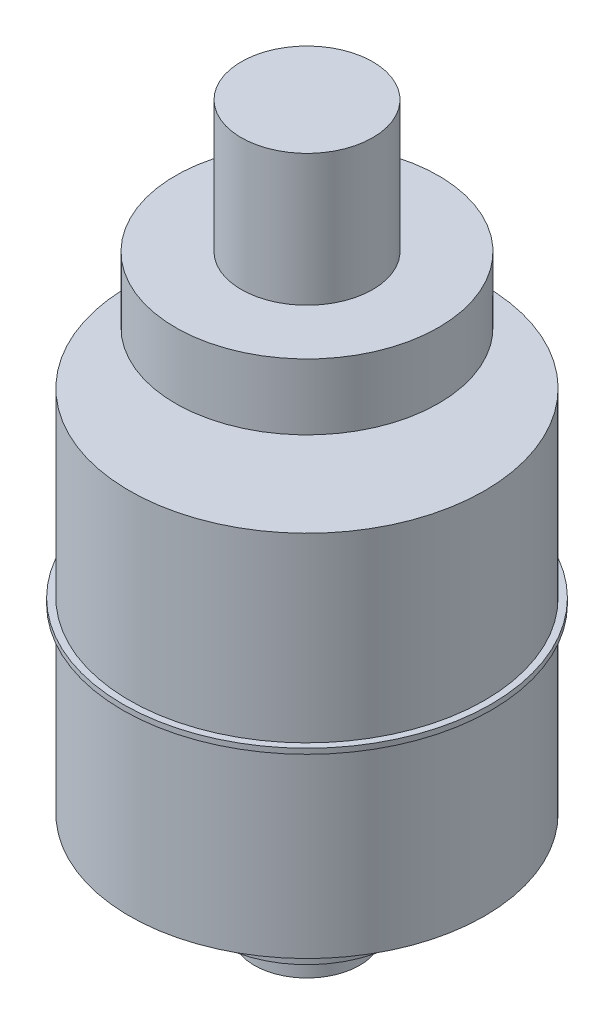
SolidWorks part; units mm, degrees
material "LY12#"
ref_plane "Front Plane" through (0, 0, 0) normal (0, 0, 1) x (1, 0, 0)
ref_plane "Top Plane" through (0, 0, 0) normal (0, 1, 0) x (1, 0, 0)
ref_plane "Right Plane" through (0, 0, 0) normal (1, 0, 0) x (0, 0, -1)
sketch "Sketch1" plane through (0, 0, 0) normal (0, 0, 1) x (1, 0, 0)
  line L0 (0, 0) -> (0, 55) construction
  line L1 (0, 55) -> (-5, 55)
  line L2 (-5, 55) -> (-5, 45)
  line L3 (-5, 45) -> (-10, 45)
  line L4 (-10, 45) -> (-10, 40)
  line L5 (-10, 40) -> (-4, 40)
  line L6 (-4, 40) -> (-4, 36)
  line L7 (-4, 36) -> (-14, 36)
  line L8 (-14, 36) -> (-14, 8)
  line L9 (-14, 8) -> (-4, 8)
  line L10 (-4, 8) -> (-4, 4)
  line L11 (-4, 4) -> (-7, 4)
  line L12 (-7, 4) -> (-7, 3)
  line L13 (-7, 3) -> (-4, 3)
  line L14 (-4, 3) -> (-4, 0)
  line L15 (-4, 0) -> (0, 0)
  line L16 (0, 0) -> (0, 55)
  line L17 (-13.5, 36) -> (-13.5, 22.2)
  line L18 (-13.5, 22.2) -> (-14, 22.2)
  line L19 (-14, 21.8) -> (-13.5, 21.8)
  line L20 (-13.5, 21.8) -> (-13.5, 8)
  line L21 (-14, 22) -> (0, 22) construction
  dimension "D1" = 10
  dimension "D2" = 10
  dimension "D3" = 5
  dimension "D4" = 20
  dimension "D5" = 45
  dimension "D6" = 8
  dimension "D7" = 3
  dimension "D8" = 1
  dimension "D9" = 28
  dimension "D10" = 4
  dimension "D11" = 28
  dimension "D12" = 14
  dimension "D13" = 4
  dimension "D14" = 0.2
  dimension "D15" = 0.2
  dimension "D16" = 0.5
  dimension "D17" = 0.5
revolve "Revolve1" add sketch "Sketch1" angle 360 about L0
